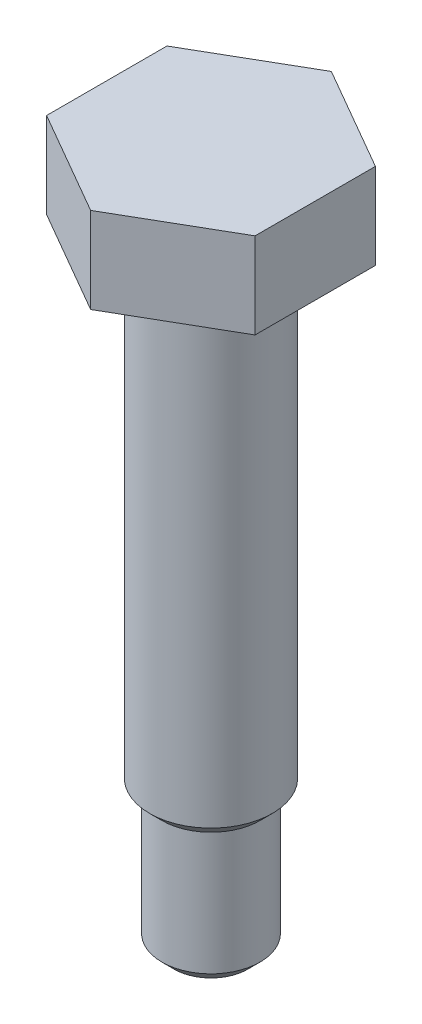
from build123d import *

# Parameters (mm, degrees)
EXTRUDE_1_DEPTH = 7
CHAMFER_1_SIZE  = 1
FILLET_1_R      = 0.5


with BuildPart() as part:
    # 草图1 → 凸台-拉伸1 (new body)
    with BuildSketch(Plane(origin=(0, 0, 0), x_dir=(1, 0, 0), z_dir=(0, 1, 0))):
        Polygon((0, 9.814954576), (-8.5, 4.907477288), (-8.5, -4.907477288), (0, -9.814954576), (8.5, -4.907477288), (8.5, 4.907477288), align=None)
    extrude(amount=EXTRUDE_1_DEPTH)

    # 草图2 → 旋转1 (revolve)
    with BuildSketch(Plane.XY, mode=Mode.PRIVATE) as revolve_1_sk:
        Polygon((0, 0), (0, -50), (4, -50), (4, -39), (5, -38), (5, 0), align=None)
    revolve(revolve_1_sk.sketch.rotate(Axis((0, 0, 0), (0, -1, 0)), 90), axis=Axis((0, 0, 0), (0, -1, 0)))

    # 倒角1
    chamfer_1_edges = [part.edges().sort_by_distance(p)[0] for p in [
        (0, -50, -4),
    ]]
    chamfer(chamfer_1_edges, length=CHAMFER_1_SIZE)

    # 圆角1
    fillet_1_edges = [part.edges().sort_by_distance(p)[0] for p in [
        (0, 0, -5),
    ]]
    fillet(fillet_1_edges, radius=FILLET_1_R)


solid = part.part
